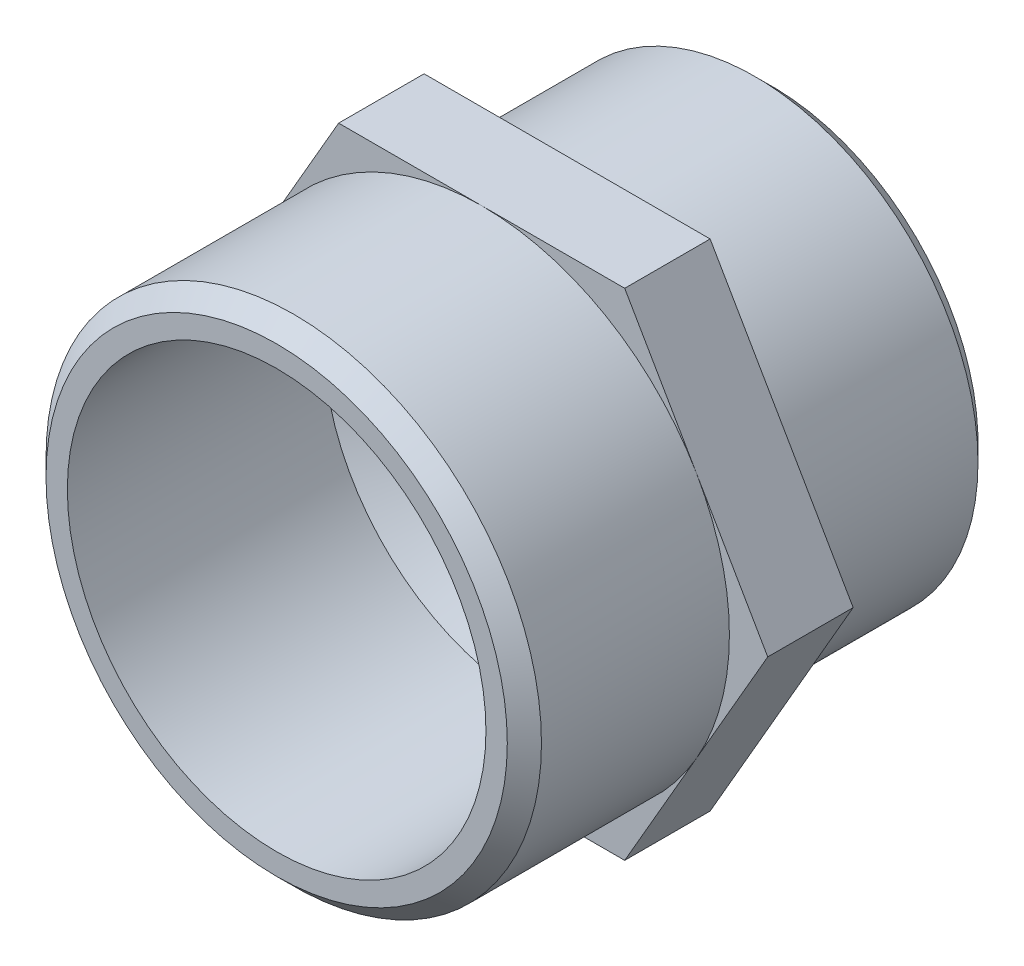
from build123d import *

# Parameters (mm, degrees)
EXTRUDE_1_DEPTH          = 2.5
SKETCH_4_R               = 13.05
EXTRUDE_3_DEPTH          = 12
CUT_EXTRUDE_2_REACH      = 29.921
SKETCH_5_R               = 9
SKETCH_6_R               = 14.5
SKETCH_6_R_2             = 9
EXTRUDE_4_DEPTH          = 12
HOLE_WIZARD_G3_4_1_D     = 24.5
HOLE_WIZARD_G3_4_1_DEPTH = 15
HOLE_WIZARD_G3_4_1_TIP   = 7.360542583
CHAMFER_1_SIZE           = 1


with BuildPart() as part:
    # 草图1 → 凸台-拉伸1 (new, symmetric)
    with BuildSketch(Plane.XY):
        Polygon((16.743157806, 0), (8.371578903, 14.5), (-8.371578903, 14.5), (-16.743157806, 0), (-8.371578903, -14.5), (8.371578903, -14.5), align=None)
    extrude(amount=EXTRUDE_1_DEPTH, both=True)

    # 草图4 → 凸台-拉伸3 (add)
    with BuildSketch(Plane(origin=(0, 0, -2.5), x_dir=(-1, 0, 0), z_dir=(0, 0, -1))):
        Circle(SKETCH_4_R)
    extrude(amount=EXTRUDE_3_DEPTH)

    # 草图5 → 切除-拉伸2 (cut, up to next)
    with BuildSketch(Plane(origin=(0, 0, -14.5), x_dir=(-1, 0, 0), z_dir=(0, 0, -1)), mode=Mode.PRIVATE) as cut_extrude_2_sk1:
        Circle(SKETCH_5_R)
    cut_extrude_2_tool1 = extrude(cut_extrude_2_sk1.sketch, amount=-CUT_EXTRUDE_2_REACH, mode=Mode.PRIVATE) & part.part
    add(cut_extrude_2_tool1.solids().sort_by_distance((0, 0, -14.5))[0], mode=Mode.SUBTRACT)

    # 草图6 → 凸台-拉伸4 (add)
    with BuildSketch(Plane.XY.offset(2.5)):
        with Locations(Location((0, 0, 0), (0, 0, 150))):
            Circle(SKETCH_6_R)
        with Locations(Location((0, 0, 0), (0, 0, 180))):
            Circle(SKETCH_6_R_2, mode=Mode.SUBTRACT)
    extrude(amount=EXTRUDE_4_DEPTH)

    # G3/4 螺纹孔1
    with Locations(Plane.XY.offset(14.5)):
        with Locations((0, 0)):
            Hole(HOLE_WIZARD_G3_4_1_D / 2, depth=HOLE_WIZARD_G3_4_1_DEPTH)
            with Locations((0, 0, -(HOLE_WIZARD_G3_4_1_DEPTH + HOLE_WIZARD_G3_4_1_TIP / 2))):  # 118° drill point
                Cone(0, HOLE_WIZARD_G3_4_1_D / 2, HOLE_WIZARD_G3_4_1_TIP, mode=Mode.SUBTRACT)

    # 倒角1
    chamfer_1_edges = [part.edges().sort_by_distance(p)[0] for p in [
        (13.05, 0, -14.5),
        (12.557368355, -7.25, 14.5),
    ]]
    chamfer(chamfer_1_edges, length=CHAMFER_1_SIZE)


solid = part.part
